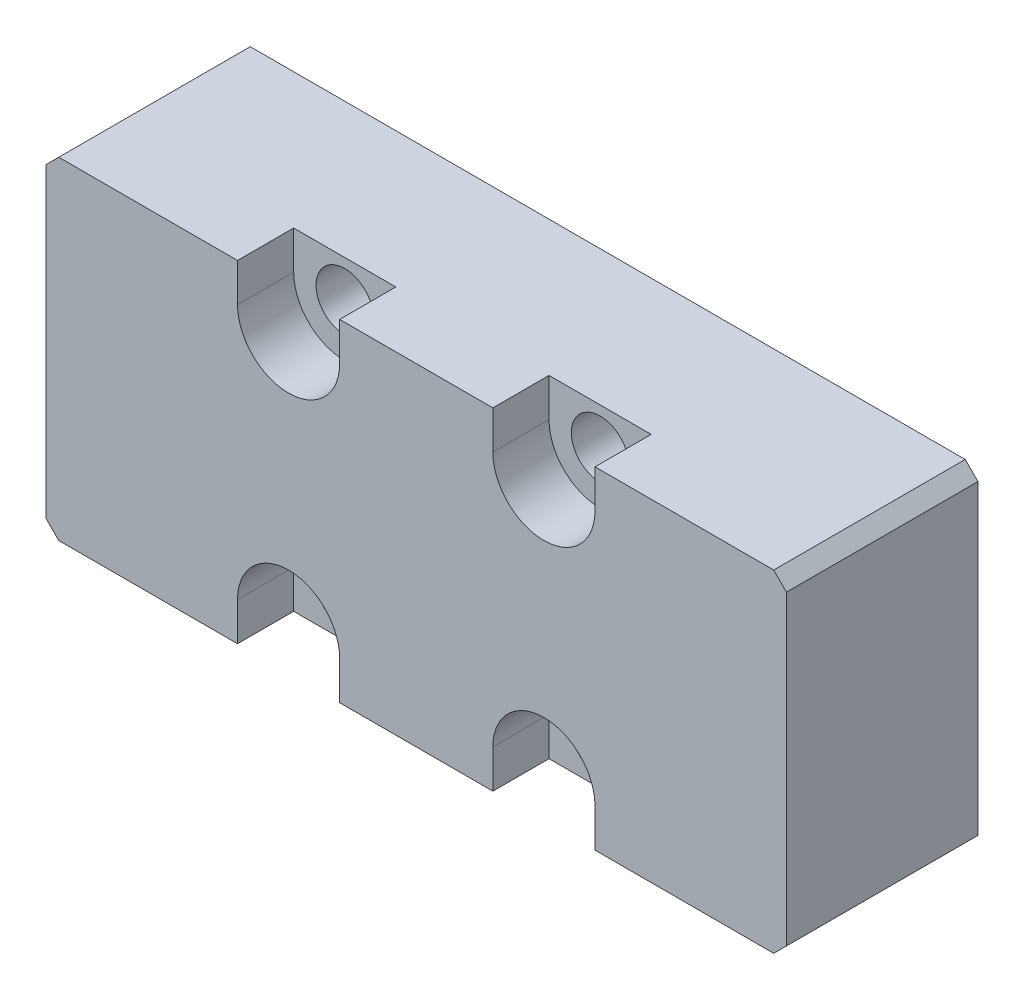
from build123d import *

# Parameters (mm, degrees)
SKETCH1_W                                           = 58
SKETCH1_H                                           = 26
BOSS_EXTRUDE1_DEPTH                                 = 7.5
CBORE_FOR_M4_HEX_SOCKET_HEAD_CAP_SCREW1_D           = 4.5
CBORE_FOR_M4_HEX_SOCKET_HEAD_CAP_SCREW1_CBORE_D     = 8
CBORE_FOR_M4_HEX_SOCKET_HEAD_CAP_SCREW1_CBORE_DEPTH = 4.4
SKETCH6_W                                           = 8
SKETCH6_H                                           = 3
CUT_EXTRUDE1_DEPTH                                  = 4.4
BLIND_PIN_HOLE1_SIZE_MM_D                           = 5
BLIND_PIN_HOLE1_SIZE_MM_DEPTH                       = 2
BLIND_PIN_HOLE1_SIZE_MM_TIP                         = 1.502151548
CHAMFER1_SIZE                                       = 1


with BuildPart() as part:
    # Sketch1 → Boss-Extrude1 (new, symmetric)
    with BuildSketch(Plane.XY):
        Rectangle(SKETCH1_W, SKETCH1_H)
    extrude(amount=BOSS_EXTRUDE1_DEPTH, both=True)

    # CBORE for M4 Hex Socket Head Cap Screw1 (through all)
    with Locations(Plane.XY.offset(7.5)):
        with Locations((-10, 10), (-10, -10), (10, -10), (10, 10)):
            CounterBoreHole(CBORE_FOR_M4_HEX_SOCKET_HEAD_CAP_SCREW1_D / 2, CBORE_FOR_M4_HEX_SOCKET_HEAD_CAP_SCREW1_CBORE_D / 2, CBORE_FOR_M4_HEX_SOCKET_HEAD_CAP_SCREW1_CBORE_DEPTH)

    # Sketch6 → Cut-Extrude1 (cut)
    with BuildSketch(Plane.XY.offset(7.5)):
        with Locations((-10, 11.5)):
            Rectangle(SKETCH6_W, SKETCH6_H)
        with Locations((10, 11.5)):
            Rectangle(SKETCH6_W, SKETCH6_H)
    cut_extrude1 = extrude(amount=-CUT_EXTRUDE1_DEPTH, mode=Mode.SUBTRACT)

    # Mirror1: Cut-Extrude1 across plane
    add(cut_extrude1.mirror(Plane.ZX), mode=Mode.SUBTRACT)

    # Blind Pin Hole1 (size mm)
    with Locations(Plane(origin=(0, 0, -7.5), x_dir=(-1, 0, 0), z_dir=(0, 0, -1))):
        with Locations((-12.5, 0), (12.5, 0)):
            Hole(BLIND_PIN_HOLE1_SIZE_MM_D / 2, depth=BLIND_PIN_HOLE1_SIZE_MM_DEPTH)
            with Locations((0, 0, -(BLIND_PIN_HOLE1_SIZE_MM_DEPTH + BLIND_PIN_HOLE1_SIZE_MM_TIP / 2))):  # 118° drill point
                Cone(0, BLIND_PIN_HOLE1_SIZE_MM_D / 2, BLIND_PIN_HOLE1_SIZE_MM_TIP, mode=Mode.SUBTRACT)

    # Chamfer1
    chamfer1_edges = [part.edges().sort_by_distance(p)[0] for p in [
        (29, -13, 0),
        (-29, -13, 0),
        (-29, 13, 0),
        (29, 13, 0),
    ]]
    chamfer(chamfer1_edges, length=CHAMFER1_SIZE)


solid = part.part
